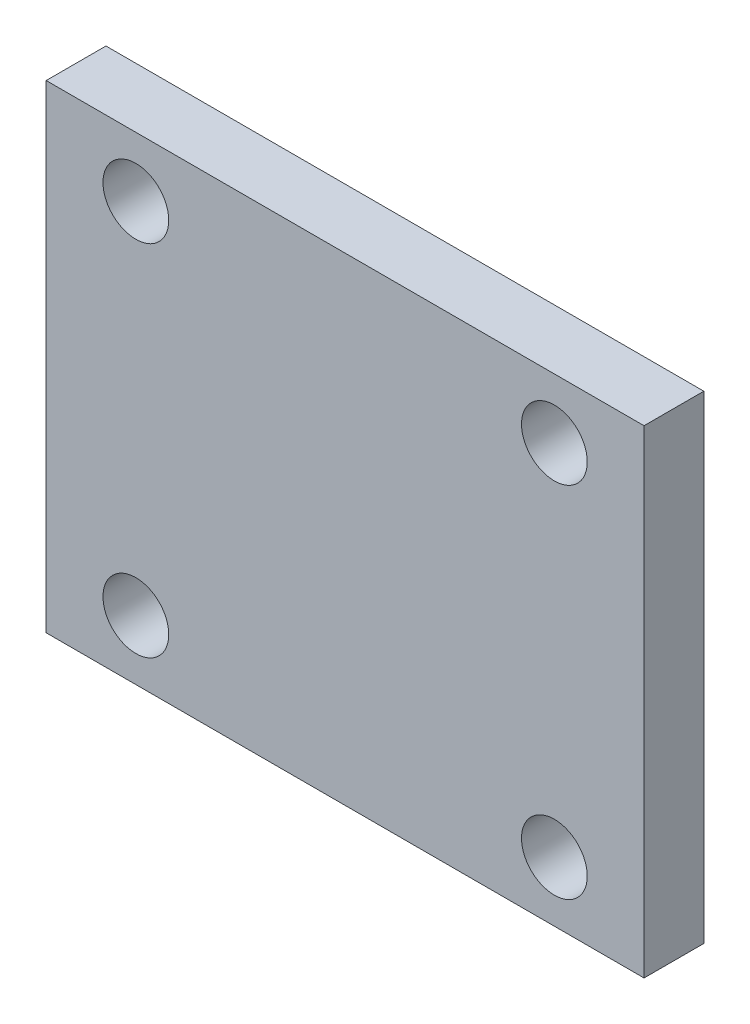
from build123d import *

# Parameters (mm, degrees)
SKETCH_1_W      = 100
SKETCH_1_H      = 80
SKETCH_1_R      = 5.5
EXTRUDE_1_DEPTH = 10


with BuildPart() as part:
    # 草图1 → 凸台-拉伸1 (new body)
    with BuildSketch(Plane.XY):
        Rectangle(SKETCH_1_W, SKETCH_1_H)
        with Locations((-35, 30)):
            Circle(SKETCH_1_R, mode=Mode.SUBTRACT)
        with Locations((-35, -30)):
            Circle(SKETCH_1_R, mode=Mode.SUBTRACT)
        with Locations((35, -30)):
            Circle(SKETCH_1_R, mode=Mode.SUBTRACT)
        with Locations((35, 30)):
            Circle(SKETCH_1_R, mode=Mode.SUBTRACT)
    extrude(amount=EXTRUDE_1_DEPTH)


solid = part.part
